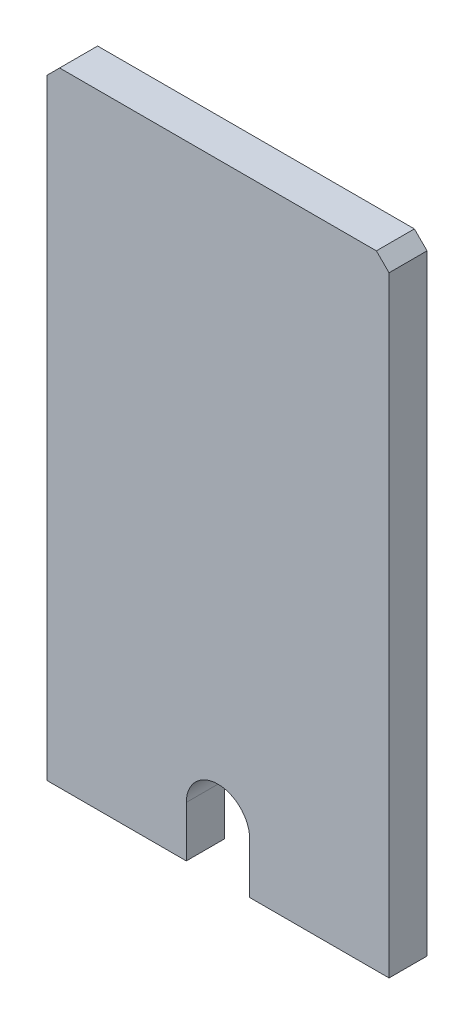
SolidWorks part; units mm, degrees
material "Q235"
ref_plane "Front Plane" through (0, 0, 0) normal (0, 0, 1) x (1, 0, 0)
ref_plane "Top Plane" through (0, 0, 0) normal (0, 1, 0) x (1, 0, 0)
ref_plane "Right Plane" through (0, 0, 0) normal (1, 0, 0) x (0, 0, -1)
sketch "Sketch1" plane through (0, 0, 0) normal (0, 0, 1) x (1, 0, 0)
  line L0 (110, 0) -> (110, 40)
  line L1 (0, 0) -> (110, 0)
  line L2 (0, 0) -> (0, 482)
  line L3 (10, 492) -> (260, 492)
  line L4 (270, 0) -> (270, 482)
  line L5 (160, 40) -> (160, 0)
  line L6 (160, 0) -> (270, 0)
  line L7 (0, 482) -> (10, 492)
  line L8 (260, 492) -> (270, 482)
  arc A0 (110, 40) -> (160, 40) centre (135, 40) cw
  point P1 (270, 492)
  point P2 (0, 492)
  dimension "D3" = 135
  dimension "D5" = 25
  dimension "D1" = 492
  dimension "D2" = 270
  dimension "D4" = 40
extrude "Boss-Extrude1" add sketch "Sketch1" along normal blind 30
